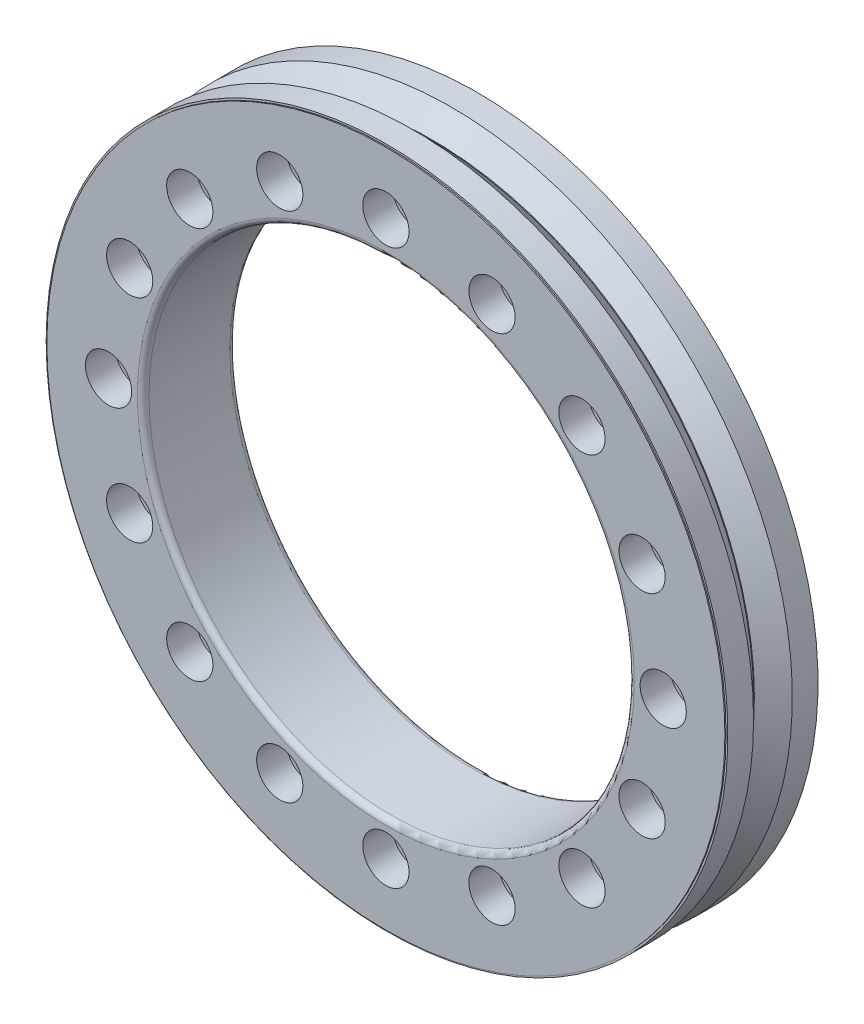
SolidWorks part; units mm, degrees
ref_plane "前视基准面" through (0, 0, 0) normal (0, 0, 1) x (1, 0, 0)
ref_plane "上视基准面" through (0, 0, 0) normal (0, 1, 0) x (1, 0, 0)
ref_plane "右视基准面" through (0, 0, 0) normal (1, 0, 0) x (0, 0, -1)
sketch "草图1" plane through (0, 0, 0) normal (0, 0, 1) x (1, 0, 0)
  circle A0 centre (0, 0) radius 105
  circle A1 centre (0, 0) radius 147.5
  dimension "D1" = 210
  dimension "D2" = 42.5
extrude "凸台-拉伸1" add sketch "草图1" along normal mid plane 40
hole_wizard "打孔尺寸(%根据)内六角圆柱头螺钉的类型2" positions "草图2" profile "草图3" counterbore size "M5" standard "GB" end condition through all
sketch "草图2" plane through (0, 0, 20) normal (0, 0, 1) x (1, 0, 0)
  line L0 (0, 16.6318) -> (0, -17.0153) construction
  point P0 (0, 120)
  dimension "D1" = 120
sketch "草图3" plane through (0, 120, 20) normal (1, 0, 0) x (0, -1, 0)
  line L0 (0, 0) -> (0, 40)
  line L1 (0, 40) -> (7, 40)
  line L3 (7, 40) -> (7, 13)
  line L4 (7, 13) -> (10, 13)
  line L5 (10, 13) -> (10, 0)
  line L7 (10, 0) -> (0, 0)
  line L11 (0, -6.35) -> (0, 107.95) construction
  dimension "通孔孔直径" = 14
  dimension "通孔孔深度" = 40
  dimension "柱形沉头孔直径" = 20
  dimension "柱形沉头孔深度" = 13
pattern_circular "阵列(圆周)1" count 16 over 360 about axis through (0, 0, 0) along (0, 0, 1) of "打孔尺寸(%根据)内六角圆柱头螺钉的类型2"
sketch "草图5" plane through (0, 0, 0) normal (0, 1, 0) x (1, 0, 0)
  line L0 (0, 0) -> (20.3926, 0) construction
  line L1 (139.2915, 0.1768) -> (147.6, 8.4853)
  line L2 (147.6, 8.4853) -> (147.6, -8.4853)
  line L3 (147.6, -8.4853) -> (139.2915, -0.1768)
  line L4 (147.5, -20) -> (147.5, 20) construction
  arc A0 (139.2915, 0.1768) -> (139.2915, -0.1768) centre (139.1147, 0) ccw
  dimension "D3" = 0.5
  dimension "D1" = 12
  dimension "D2" = 0.1
  dimension "D4" = 45
ref_axis "基准轴1" through (0, 0, 20) along (0, 0, -1)
revolve "切除-旋转1" cut sketch "草图5" angle 360 about axis through (0, 0, 20) along (0, 0, -1)
sketch "草图6" plane through (0, 0, -20) normal (0, 0, -1) x (-1, 0, 0)
  circle A0 centre (0, 0) radius 146.7
  circle A1 centre (0, 0) radius 147.5
  circle A2 centre (0, 0) radius 147.5 construction
  dimension "D2" = 0.8
extrude "切除-拉伸1" cut sketch "草图6" against normal blind 0.5
mirror "镜向1" about plane through (0, 0, 0) normal (0, 0, 1) of "切除-拉伸1"
fillet "圆角1" radius 2.5 2 edges at (105, 0, 20) (105, 0, -20)
